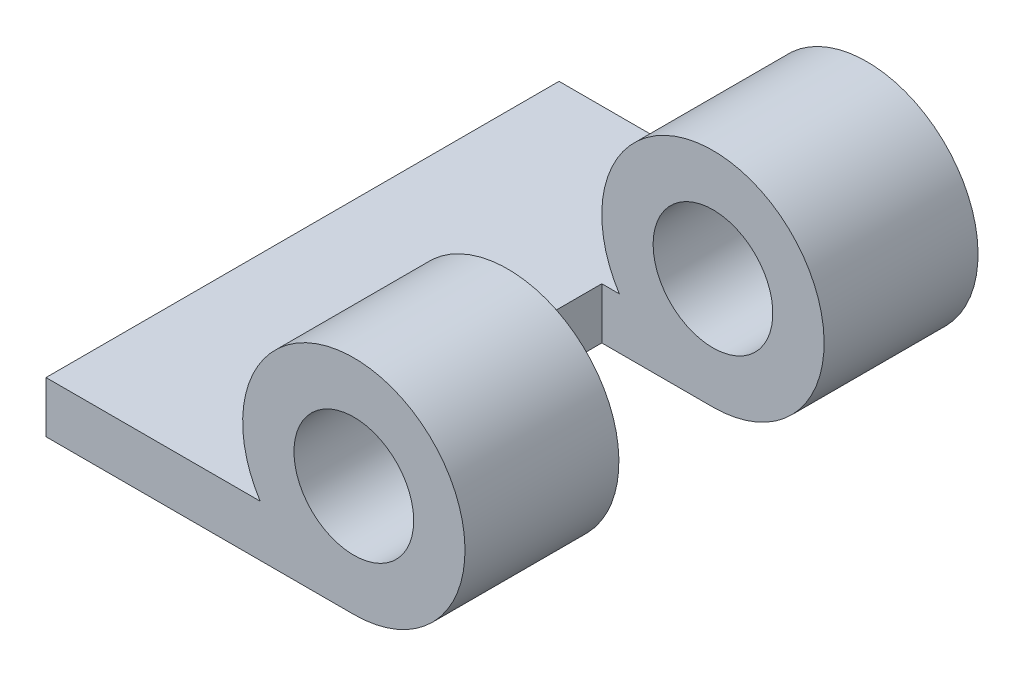
from build123d import *

# Parameters (mm, degrees)
SKETCH_1_R          = 3.5
EXTRUDE_1_DEPTH     = 30
SKETCH_2_W          = 19.333042973
SKETCH_2_H          = 12
CUT_EXTRUDE_1_DEPTH = 15


with BuildPart() as part:
    # 草图1 → 凸台-拉伸1 (new body)
    with BuildSketch(Plane.XY):
        with BuildLine():
            Line((-9, 1.5), (3.522774425, 1.5))
            ThreePointArc((3.522774425, 1.5), (12.122498999, 10.700877125), (9, -1.5))
            Line((9, -1.5), (-9, -1.5))
            Line((-9, -1.5), (-9, 1.5))
        make_face()
        with Locations((9, 5)):
            Circle(SKETCH_1_R, mode=Mode.SUBTRACT)
    extrude(amount=EXTRUDE_1_DEPTH)

    # 草图2 → 切除-拉伸1 (cut, symmetric)
    with BuildSketch(Plane(origin=(0, 0, 0), x_dir=(1, 0, 0), z_dir=(0, 1, 0))):
        with Locations((12.166521487, -15)):
            Rectangle(SKETCH_2_W, SKETCH_2_H)
    extrude(amount=CUT_EXTRUDE_1_DEPTH, both=True, mode=Mode.SUBTRACT)


solid = part.part
